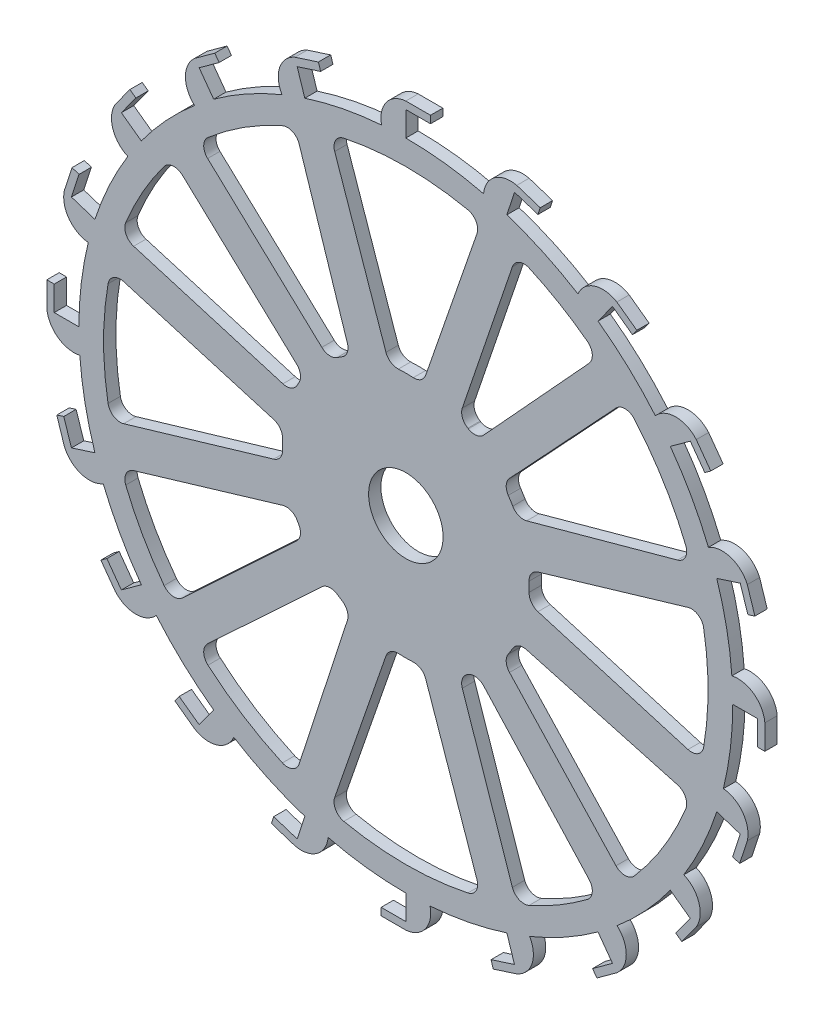
SolidWorks part; units mm, degrees
material "Q235A"
ref_plane "前视基准面" through (0, 0, 0) normal (0, 0, 1) x (1, 0, 0)
ref_plane "上视基准面" through (0, 0, 0) normal (0, 1, 0) x (1, 0, 0)
ref_plane "右视基准面" through (0, 0, 0) normal (1, 0, 0) x (0, 0, -1)
sketch "草图1" plane through (0, 0, 0) normal (0, 0, 1) x (1, 0, 0)
  line B0 (115.4655, -40.9141) -> (25.2954, -16.1289)
  line B1 (88.8732, -84.3078) -> (25.2954, -16.1289)
  line B2 (-30.6464, 118.6046) -> (0, 30)
  line B3 (30.6464, 118.6046) -> (0, 30)
  line B4 (-119.6013, -26.4909) -> (-30, 0)
  line B5 (-119.6013, 26.4909) -> (-30, 0)
  line B6 (30.6464, -118.6046) -> (0, -30)
  line B7 (-30.6464, -118.6046) -> (0, -30)
  line B8 (-115.4672, 40.9094) -> (-26.3476, 14.3458)
  line B9 (-94.5377, 77.903) -> (-26.3476, 14.3458)
  line B10 (-94.5377, -77.903) -> (-26.3476, -14.3458)
  line B11 (-115.4672, -40.9094) -> (-26.3476, -14.3458)
  line B12 (-44.9165, -113.9682) -> (-16.1091, -25.3081)
  line B13 (-84.3077, -88.8733) -> (-16.1091, -25.3081)
  line B14 (77.9043, -94.5366) -> (15, -25.9808)
  line B15 (44.9136, -113.9694) -> (15, -25.9808)
  line B16 (88.8732, 84.3078) -> (25.2954, 16.1289)
  line B17 (115.4655, 40.9141) -> (25.2954, 16.1289)
  line B18 (119.6013, 26.4909) -> (30, 0)
  line B19 (119.6013, -26.4909) -> (30, 0)
  line B20 (44.9136, 113.9694) -> (15, 25.9808)
  line B21 (77.9043, 94.5366) -> (15, 25.9808)
  line B22 (-84.3077, 88.8733) -> (-16.1091, 25.3081)
  line B23 (-44.9165, 113.9682) -> (-16.1091, 25.3081)
  line B24 (0, 145.5) -> (10, 145.5)
  line B25 (10, 145.5) -> (10, 142.5)
  line B26 (10, 142.5) -> (0, 142.5)
  line B27 (0, 132.5) -> (0, 142.5)
  line B28 (-44.962, 138.3787) -> (-35.4514, 141.4689)
  line B29 (-35.4514, 141.4689) -> (-34.5244, 138.6157)
  line B30 (-34.5244, 138.6157) -> (-44.0349, 135.5256)
  line B31 (-40.9448, 126.015) -> (-44.0349, 135.5256)
  line B32 (-85.5228, 117.712) -> (-77.4326, 123.5898)
  line B33 (-77.4326, 123.5898) -> (-75.6692, 121.1628)
  line B34 (-75.6692, 121.1628) -> (-83.7594, 115.2849)
  line B35 (-77.8815, 107.1948) -> (-83.7594, 115.2849)
  line B36 (-117.712, 85.5228) -> (-111.8341, 93.6129)
  line B37 (-111.8341, 93.6129) -> (-109.4071, 91.8496)
  line B38 (-109.4071, 91.8496) -> (-115.2849, 83.7594)
  line B39 (-107.1948, 77.8815) -> (-115.2849, 83.7594)
  line B40 (-138.3787, 44.962) -> (-135.2886, 54.4725)
  line B41 (-135.2886, 54.4725) -> (-132.4354, 53.5455)
  line B42 (-132.4354, 53.5455) -> (-135.5256, 44.0349)
  line B43 (-126.015, 40.9448) -> (-135.5256, 44.0349)
  line B44 (-145.5, 0) -> (-145.5, 10)
  line B45 (-145.5, 10) -> (-142.5, 10)
  line B46 (-142.5, 10) -> (-142.5, 0)
  line B47 (-132.5, 0) -> (-142.5, 0)
  line B48 (-138.3787, -44.962) -> (-141.4689, -35.4514)
  line B49 (-141.4689, -35.4514) -> (-138.6157, -34.5244)
  line B50 (-138.6157, -34.5244) -> (-135.5256, -44.0349)
  line B51 (-126.015, -40.9448) -> (-135.5256, -44.0349)
  line B52 (-117.712, -85.5228) -> (-123.5898, -77.4326)
  line B53 (-123.5898, -77.4326) -> (-121.1628, -75.6692)
  line B54 (-121.1628, -75.6692) -> (-115.2849, -83.7594)
  line B55 (-107.1948, -77.8815) -> (-115.2849, -83.7594)
  line B56 (-85.5228, -117.712) -> (-93.6129, -111.8341)
  line B57 (-93.6129, -111.8341) -> (-91.8496, -109.4071)
  line B58 (-91.8496, -109.4071) -> (-83.7594, -115.2849)
  line B59 (-77.8815, -107.1948) -> (-83.7594, -115.2849)
  line B60 (-44.962, -138.3787) -> (-54.4725, -135.2886)
  line B61 (-54.4725, -135.2886) -> (-53.5455, -132.4354)
  line B62 (-53.5455, -132.4354) -> (-44.0349, -135.5256)
  line B63 (-40.9448, -126.015) -> (-44.0349, -135.5256)
  line B64 (0, -145.5) -> (-10, -145.5)
  line B65 (-10, -145.5) -> (-10, -142.5)
  line B66 (-10, -142.5) -> (0, -142.5)
  line B67 (0, -132.5) -> (0, -142.5)
  line B68 (44.962, -138.3787) -> (35.4514, -141.4689)
  line B69 (35.4514, -141.4689) -> (34.5244, -138.6157)
  line B70 (34.5244, -138.6157) -> (44.0349, -135.5256)
  line B71 (40.9448, -126.015) -> (44.0349, -135.5256)
  line B72 (85.5228, -117.712) -> (77.4326, -123.5898)
  line B73 (77.4326, -123.5898) -> (75.6692, -121.1628)
  line B74 (75.6692, -121.1628) -> (83.7594, -115.2849)
  line B75 (77.8815, -107.1948) -> (83.7594, -115.2849)
  line B76 (117.712, -85.5228) -> (111.8341, -93.6129)
  line B77 (111.8341, -93.6129) -> (109.4071, -91.8496)
  line B78 (109.4071, -91.8496) -> (115.2849, -83.7594)
  line B79 (107.1948, -77.8815) -> (115.2849, -83.7594)
  line B80 (138.3787, -44.962) -> (135.2886, -54.4725)
  line B81 (135.2886, -54.4725) -> (132.4354, -53.5455)
  line B82 (132.4354, -53.5455) -> (135.5256, -44.0349)
  line B83 (126.015, -40.9448) -> (135.5256, -44.0349)
  line B84 (145.5, 0) -> (145.5, -10)
  line B85 (145.5, -10) -> (142.5, -10)
  line B86 (142.5, -10) -> (142.5, 0)
  line B87 (132.5, 0) -> (142.5, 0)
  line B88 (138.3787, 44.962) -> (141.4689, 35.4514)
  line B89 (141.4689, 35.4514) -> (138.6157, 34.5244)
  line B90 (138.6157, 34.5244) -> (135.5256, 44.0349)
  line B91 (126.015, 40.9448) -> (135.5256, 44.0349)
  line B92 (117.712, 85.5228) -> (123.5898, 77.4326)
  line B93 (123.5898, 77.4326) -> (121.1628, 75.6692)
  line B94 (121.1628, 75.6692) -> (115.2849, 83.7594)
  line B95 (107.1948, 77.8815) -> (115.2849, 83.7594)
  line B96 (85.5228, 117.712) -> (93.6129, 111.8341)
  line B97 (93.6129, 111.8341) -> (91.8496, 109.4071)
  line B98 (91.8496, 109.4071) -> (83.7594, 115.2849)
  line B99 (77.8815, 107.1948) -> (83.7594, 115.2849)
  line B100 (44.962, 138.3787) -> (54.4725, 135.2886)
  line B101 (54.4725, 135.2886) -> (53.5455, 132.4354)
  line B102 (53.5455, 132.4354) -> (44.0349, 135.5256)
  line B103 (40.9448, 126.015) -> (44.0349, 135.5256)
  arc B104 (88.8732, -84.3078) -> (115.4655, -40.9141) centre (0, 0) ccw
  arc B105 (30.6464, 118.6046) -> (-30.6464, 118.6046) centre (0, 0) ccw
  arc B106 (-119.6013, 26.4909) -> (-119.6013, -26.4909) centre (0, 0) ccw
  arc B107 (-30.6464, -118.6046) -> (30.6464, -118.6046) centre (0, 0) ccw
  arc B108 (-94.5377, 77.903) -> (-115.4672, 40.9094) centre (0, 0) ccw
  arc B109 (-115.4672, -40.9094) -> (-94.5377, -77.903) centre (0, 0) ccw
  arc B110 (-84.3077, -88.8733) -> (-44.9165, -113.9682) centre (0, 0) ccw
  arc B111 (44.9136, -113.9694) -> (77.9043, -94.5366) centre (0, 0) ccw
  arc B112 (115.4655, 40.9141) -> (88.8732, 84.3078) centre (0, 0) ccw
  arc B113 (119.6013, -26.4909) -> (119.6013, 26.4909) centre (0, 0) ccw
  arc B114 (77.9043, 94.5366) -> (44.9136, 113.9694) centre (0, 0) ccw
  arc B115 (-44.9165, 113.9682) -> (-84.3077, 88.8733) centre (0, 0) ccw
  circle B116 centre (0, 0) radius 15
  arc B117 (-9.8137, 132.1361) -> (-40.9448, 126.015) centre (0, 0) ccw
  arc B118 (0, 145.5) -> (-9.8137, 132.1361) centre (0.9207, 134.5386) ccw
  arc B119 (-44.962, 138.3787) -> (-50.1657, 122.6363) centre (-40.6991, 128.2383) ccw
  arc B120 (-85.5228, 117.712) -> (-85.6071, 101.132) centre (-78.3349, 109.3852) ccw
  arc B121 (-117.712, 85.5228) -> (-112.6687, 69.7282) centre (-108.3028, 79.8247) ccw
  arc B122 (-138.3787, 44.962) -> (-128.7015, 31.4989) centre (-127.6693, 42.4504) ccw
  arc B123 (-145.5, 0) -> (-132.1361, -9.8137) centre (-134.5386, 0.9207) ccw
  arc B124 (-138.3787, -44.962) -> (-122.6363, -50.1657) centre (-128.2383, -40.6991) ccw
  arc B125 (-117.712, -85.5228) -> (-101.132, -85.6071) centre (-109.3852, -78.3349) ccw
  arc B126 (-85.5228, -117.712) -> (-69.7282, -112.6687) centre (-79.8247, -108.3028) ccw
  arc B127 (-44.962, -138.3787) -> (-31.4989, -128.7015) centre (-42.4504, -127.6693) ccw
  arc B128 (0, -145.5) -> (9.8137, -132.1361) centre (-0.9207, -134.5386) ccw
  arc B129 (44.962, -138.3787) -> (50.1657, -122.6363) centre (40.6991, -128.2383) ccw
  arc B130 (85.5228, -117.712) -> (85.6071, -101.132) centre (78.3349, -109.3852) ccw
  arc B131 (117.712, -85.5228) -> (112.6687, -69.7282) centre (108.3028, -79.8247) ccw
  arc B132 (138.3787, -44.962) -> (128.7015, -31.4989) centre (127.6693, -42.4504) ccw
  arc B133 (145.5, 0) -> (132.1361, 9.8137) centre (134.5386, -0.9207) ccw
  arc B134 (138.3787, 44.962) -> (122.6363, 50.1657) centre (128.2383, 40.6991) ccw
  arc B135 (117.712, 85.5228) -> (101.132, 85.6071) centre (109.3852, 78.3349) ccw
  arc B136 (85.5228, 117.712) -> (69.7282, 112.6687) centre (79.8247, 108.3028) ccw
  arc B137 (44.962, 138.3787) -> (31.4989, 128.7015) centre (42.4504, 127.6693) ccw
  arc B138 (31.4989, 128.7015) -> (0, 132.5) centre (0, 0) ccw
  arc B139 (69.7282, 112.6687) -> (40.9448, 126.015) centre (0, 0) ccw
  arc B140 (101.132, 85.6071) -> (77.8815, 107.1948) centre (0, 0) ccw
  arc B141 (122.6363, 50.1657) -> (107.1948, 77.8815) centre (0, 0) ccw
  arc B142 (132.1361, 9.8137) -> (126.015, 40.9448) centre (0, 0) ccw
  arc B143 (128.7015, -31.4989) -> (132.5, 0) centre (0, 0) ccw
  arc B144 (112.6687, -69.7282) -> (126.015, -40.9448) centre (0, 0) ccw
  arc B145 (85.6071, -101.132) -> (107.1948, -77.8815) centre (0, 0) ccw
  arc B146 (50.1657, -122.6363) -> (77.8815, -107.1948) centre (0, 0) ccw
  arc B147 (9.8137, -132.1361) -> (40.9448, -126.015) centre (0, 0) ccw
  arc B148 (-31.4989, -128.7015) -> (0, -132.5) centre (0, 0) ccw
  arc B149 (-69.7282, -112.6687) -> (-40.9448, -126.015) centre (0, 0) ccw
  arc B150 (-101.132, -85.6071) -> (-77.8815, -107.1948) centre (0, 0) ccw
  arc B151 (-122.6363, -50.1657) -> (-107.1948, -77.8815) centre (0, 0) ccw
  arc B152 (-132.1361, -9.8137) -> (-126.015, -40.9448) centre (0, 0) ccw
  arc B153 (-128.7015, 31.4989) -> (-132.5, 0) centre (0, 0) ccw
  arc B154 (-112.6687, 69.7282) -> (-126.015, 40.9448) centre (0, 0) ccw
  arc B155 (-85.6071, 101.132) -> (-107.1948, 77.8815) centre (0, 0) ccw
  arc B156 (-50.1657, 122.6363) -> (-77.8815, 107.1948) centre (0, 0) ccw
sketch_block_instance "转片1-1"
sketch_block "转片1"
extrude "凸台-拉伸1" add sketch "草图1" along normal blind 5
sketch "草图3" plane through (0, 0, 0) normal (0, 0, -1) x (-1, 0, 0)
  line L2 (-25.2954, -16.1289) -> (-115.4655, -40.9141)
  line L3 (-88.8732, -84.3078) -> (-25.2954, -16.1289)
  line L4 (-25.2954, -16.1289) -> (-45.106, -21.5743)
  line L5 (-39.1993, -31.039) -> (-25.2954, -16.1289)
  line L6 (0, 30) -> (30.6464, 118.6046)
  line L7 (-30.6464, 118.6046) -> (0, 30)
  line L8 (0, 30) -> (6.7588, 49.5411)
  line L9 (-6.7588, 49.5411) -> (0, 30)
  line L10 (30, 0) -> (119.6013, -26.4909)
  line L11 (119.6013, 26.4909) -> (30, 0)
  line L12 (30, 0) -> (49.661, -5.8128)
  line L13 (49.661, 5.8128) -> (30, 0)
  line L14 (0, -30) -> (-30.6464, -118.6046)
  line L15 (30.6464, -118.6046) -> (0, -30)
  line L16 (0, -30) -> (-6.7588, -49.5411)
  line L17 (6.7588, -49.5411) -> (0, -30)
  line L18 (26.3476, 14.3458) -> (115.4672, 40.9094)
  line L19 (94.5377, 77.903) -> (26.3476, 14.3458)
  line L20 (26.3476, 14.3458) -> (45.767, 20.1341)
  line L21 (41.2588, 28.2438) -> (26.3476, 14.3458)
  line L22 (26.3476, -14.3458) -> (94.5377, -77.903)
  line L23 (115.4672, -40.9094) -> (26.3476, -14.3458)
  line L24 (26.3476, -14.3458) -> (41.2588, -28.2438)
  line L25 (45.767, -20.1341) -> (26.3476, -14.3458)
  line L26 (16.1091, -25.3081) -> (44.9165, -113.9682)
  line L27 (84.3077, -88.8733) -> (16.1091, -25.3081)
  line L28 (16.1091, -25.3081) -> (22.409, -44.6972)
  line L29 (31.0248, -39.2105) -> (16.1091, -25.3081)
  line L30 (-15, -25.9808) -> (-77.9043, -94.5366)
  line L31 (-44.9136, -113.9694) -> (-15, -25.9808)
  line L32 (-15, -25.9808) -> (-28.7174, -40.9306)
  line L33 (-21.5121, -45.1357) -> (-15, -25.9808)
  line L34 (-25.2954, 16.1289) -> (-88.8732, 84.3078)
  line L35 (-115.4655, 40.9141) -> (-25.2954, 16.1289)
  line L36 (-25.2954, 16.1289) -> (-39.1993, 31.039)
  line L37 (-45.106, 21.5743) -> (-25.2954, 16.1289)
  line L38 (-30, 0) -> (-119.6013, 26.4909)
  line L39 (-119.6013, -26.4909) -> (-30, 0)
  line L40 (-30, 0) -> (-49.661, 5.8128)
  line L41 (-49.661, -5.8128) -> (-30, 0)
  line L42 (-15, 25.9808) -> (-44.9136, 113.9694)
  line L43 (-77.9043, 94.5366) -> (-15, 25.9808)
  line L44 (-15, 25.9808) -> (-21.5121, 45.1357)
  line L45 (-28.7174, 40.9306) -> (-15, 25.9808)
  line L46 (16.1091, 25.3081) -> (84.3077, 88.8733)
  line L47 (44.9165, 113.9682) -> (16.1091, 25.3081)
  line L48 (16.1091, 25.3081) -> (31.0248, 39.2105)
  line L49 (22.409, 44.6972) -> (16.1091, 25.3081)
  arc A0 (-21.5121, 45.1357) -> (-28.7174, 40.9306) centre (0, 0) ccw
  arc A1 (-115.4655, -40.9141) -> (-88.8732, -84.3078) centre (0, 0) ccw
  arc A3 (30.6464, 118.6046) -> (-30.6464, 118.6046) centre (0, 0) ccw
  arc A5 (119.6013, -26.4909) -> (119.6013, 26.4909) centre (0, 0) ccw
  arc A7 (-30.6464, -118.6046) -> (30.6464, -118.6046) centre (0, 0) ccw
  arc A9 (115.4672, 40.9094) -> (94.5377, 77.903) centre (0, 0) ccw
  arc A11 (94.5377, -77.903) -> (115.4672, -40.9094) centre (0, 0) ccw
  arc A13 (44.9165, -113.9682) -> (84.3077, -88.8733) centre (0, 0) ccw
  arc A15 (-77.9043, -94.5366) -> (-44.9136, -113.9694) centre (0, 0) ccw
  arc A17 (-88.8732, 84.3078) -> (-115.4655, 40.9141) centre (0, 0) ccw
  arc A19 (-119.6013, 26.4909) -> (-119.6013, -26.4909) centre (0, 0) ccw
  arc A21 (-44.9136, 113.9694) -> (-77.9043, 94.5366) centre (0, 0) ccw
  arc A23 (84.3077, 88.8733) -> (44.9165, 113.9682) centre (0, 0) ccw
  arc A27 (-39.1993, 31.039) -> (-45.106, 21.5743) centre (0, 0) ccw
  arc A28 (-49.661, 5.8128) -> (-49.661, -5.8128) centre (0, 0) ccw
  arc A29 (-45.106, -21.5743) -> (-39.1993, -31.039) centre (0, 0) ccw
  arc A30 (-28.7174, -40.9306) -> (-21.5121, -45.1357) centre (0, 0) ccw
  arc A31 (-6.7588, -49.5411) -> (6.7588, -49.5411) centre (0, 0) ccw
  arc A32 (22.409, -44.6972) -> (31.0248, -39.2105) centre (0, 0) ccw
  arc A33 (41.2588, -28.2438) -> (45.767, -20.1341) centre (0, 0) ccw
  arc A34 (49.661, -5.8128) -> (49.661, 5.8128) centre (0, 0) ccw
  arc A35 (45.767, 20.1341) -> (41.2588, 28.2438) centre (0, 0) ccw
  arc A36 (31.0248, 39.2105) -> (22.409, 44.6972) centre (0, 0) ccw
  arc A37 (6.7588, 49.5411) -> (-6.7588, 49.5411) centre (0, 0) ccw
  dimension "D1" = 0
  dimension "D14" = 100
  dimension "D2" = 0
  dimension "D3" = 0
  dimension "D4" = 0
  dimension "D5" = 0
  dimension "D6" = 0
  dimension "D7" = 0
  dimension "D8" = 0
  dimension "D9" = 0
  dimension "D10" = 0
  dimension "D11" = 0
  dimension "D12" = 0
extrude "凸台-拉伸2" add sketch "草图3" against normal through all
fillet "圆角1" radius 5 48 edges at (39.1993, -31.039, 2.5) (88.8732, -84.3078, 2.5) (115.4655, -40.9141, 2.5) (45.106, -21.5743, 2.5) (6.7588, 49.5411, 2.5) (30.6464, 118.6046, 2.5) (-30.6464, 118.6046, 2.5) (-6.7588, 49.5411, 2.5) (-49.661, 5.8128, 2.5) (-119.6013, 26.4909, 2.5) (-49.661, -5.8128, 2.5) (-6.7588, -49.5411, 2.5) (-30.6464, -118.6046, 2.5) (30.6464, -118.6046, 2.5) (6.7588, -49.5411, 2.5) (-41.2588, 28.2438, 2.5) (-94.5377, 77.903, 2.5) (-115.4672, 40.9094, 2.5) (-45.767, 20.1341, 2.5) (-45.767, -20.1341, 2.5) (-115.4672, -40.9094, 2.5) (-94.5377, -77.903, 2.5) (-41.2588, -28.2438, 2.5) (-31.0248, -39.2105, 2.5) (-84.3077, -88.8733, 2.5) (-44.9165, -113.9682, 2.5) (-22.409, -44.6972, 2.5) (21.5121, -45.1357, 2.5) (44.9136, -113.9694, 2.5) (77.9043, -94.5366, 2.5) (28.7174, -40.9306, 2.5) (45.106, 21.5743, 2.5) (115.4655, 40.9141, 2.5) (88.8732, 84.3078, 2.5) (39.1993, 31.039, 2.5) (49.661, -5.8128, 2.5) (119.6013, -26.4909, 2.5) (119.6013, 26.4909, 2.5) (49.661, 5.8128, 2.5) (28.7174, 40.9306, 2.5) (77.9043, 94.5366, 2.5) (44.9136, 113.9694, 2.5) (21.5121, 45.1357, 2.5) (-22.409, 44.6972, 2.5) (-44.9165, 113.9682, 2.5) (-84.3077, 88.8733, 2.5) (-31.0248, 39.2105, 2.5) (-119.6013, -26.4909, 2.5)
sketch "草图4" plane through (0, 0, 0) normal (0, 0, -1) x (-1, 0, 0)
  circle A0 centre (0, 0) radius 15 construction
  circle A1 centre (0, 0) radius 15
  circle A2 centre (0, 0) radius 15.1
  dimension "D1" = 0.1
extrude "切除-拉伸1" cut sketch "草图4" against normal through all
